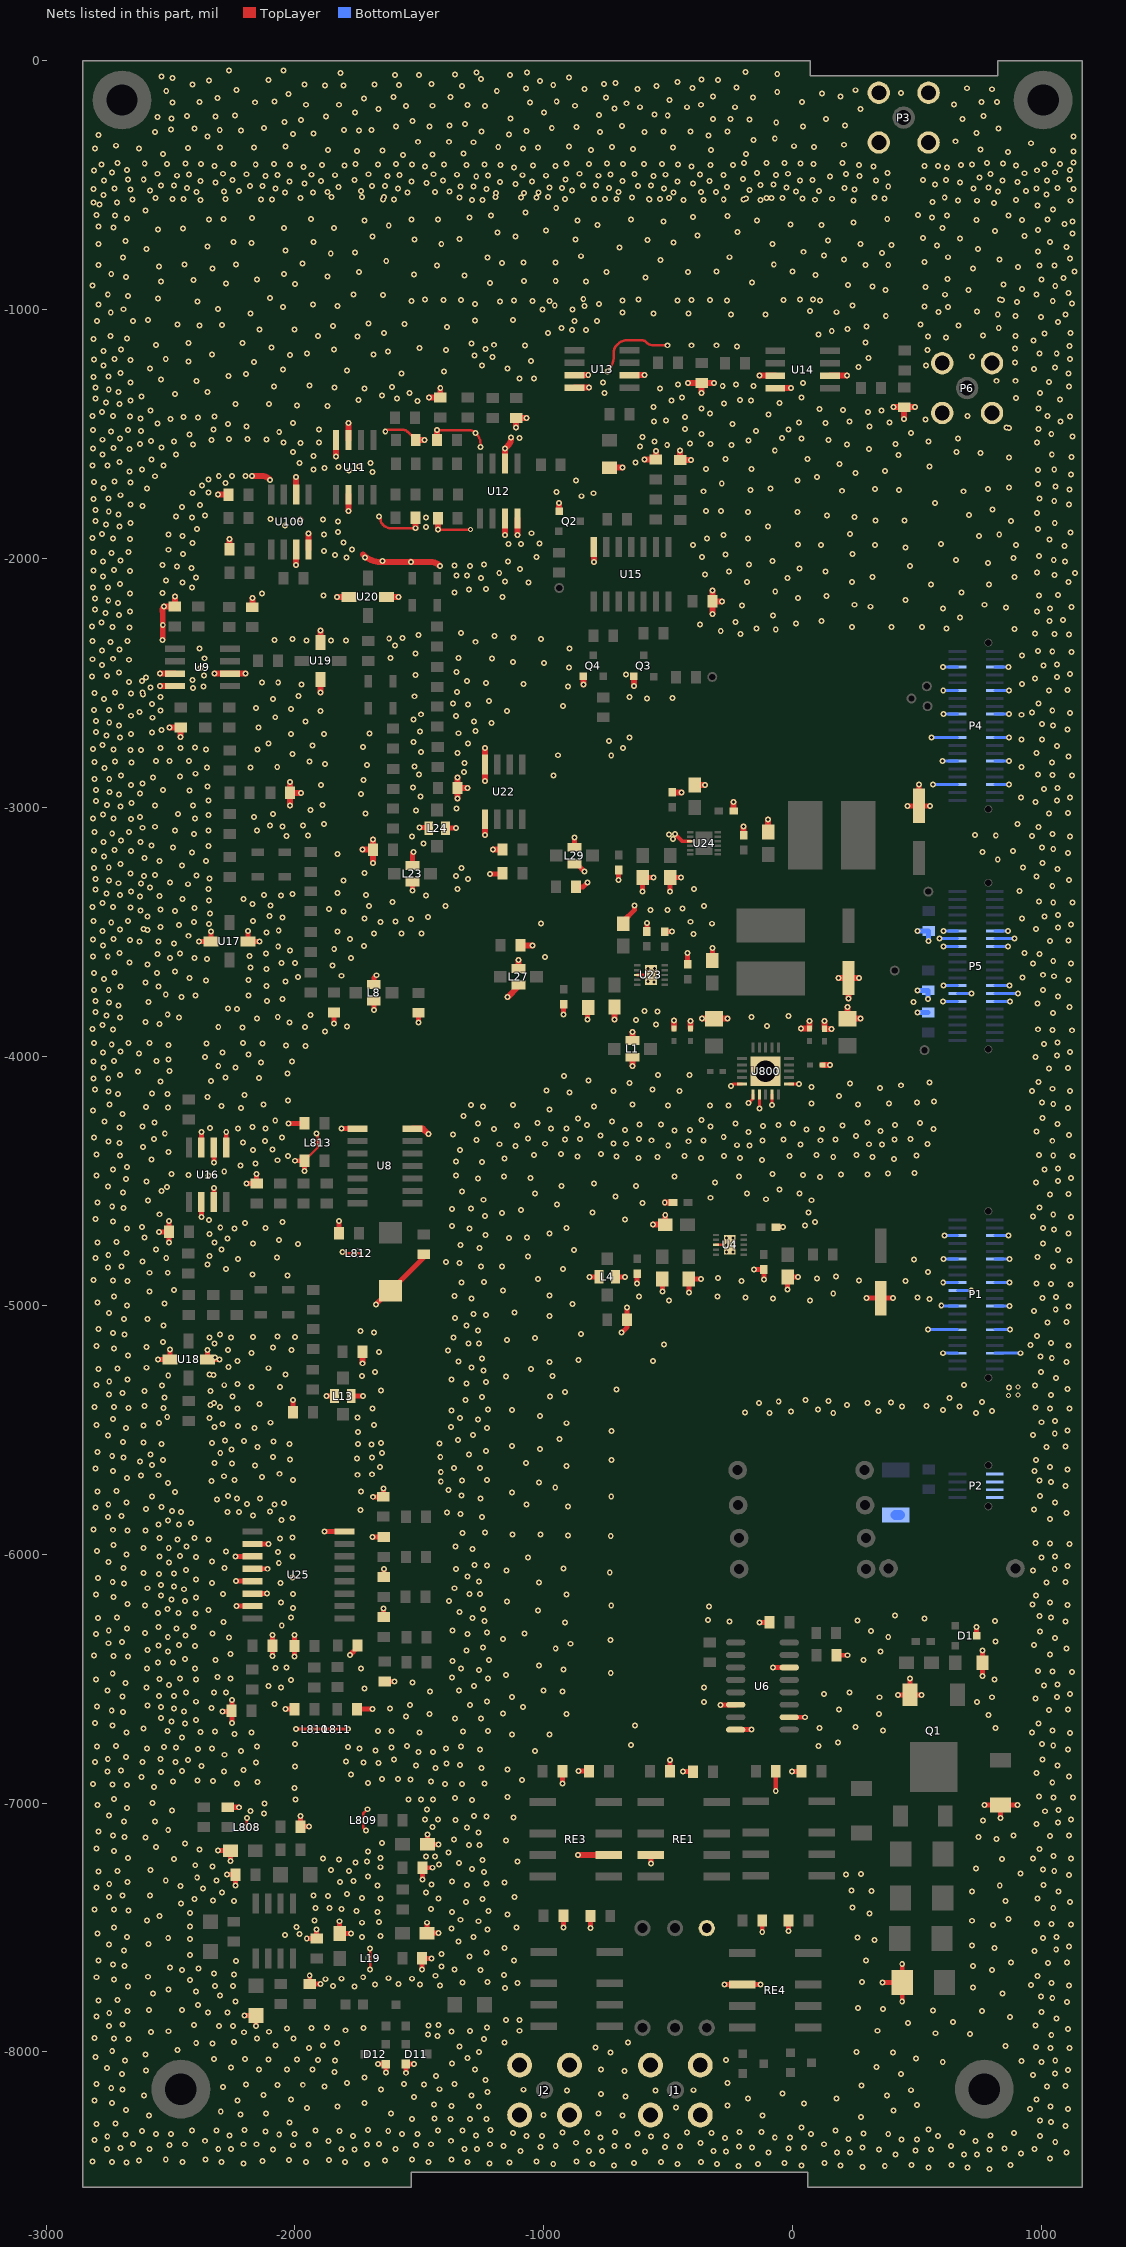
[diagram p0: the nets of this part, all layers, seen from the top]
# Altium PCB MISC109560.PcbDoc (part 4 of 7)
Units mil, origin at the board's own origin, x right, y up, seen from the top; angles counter-clockwise.
Board outline 4015.75 x 8543.31 mil, 4 copper layers (TopLayer, GND, SIG3, BottomLayer); 280 components, 173 nets, 936 pads, 3695 vias.

## Via types
v1: diameter 24, hole 12, TopLayer to BottomLayer, 3659 vias
v2: diameter 20, hole 12, TopLayer to BottomLayer, 32 vias
v3: diameter 40, hole 20, TopLayer to BottomLayer, 4 vias

## Nets (pads, with @x,y where several pads share a name; then routed paths per layer and width w, separated by ;. In a path a pad name is that pad's centre, name@x,y a point inside that pad or via, vN(x,y) a via of type N, cw(c..) or ccw(c..) an arc to the next point about the centre after c; other vN are vias at no path point) (continued)
GND: (continued)
  other v1: 790,-8471 545,-8464 702,-8464 280,-8463 370,-8459 -217,-8458 -717,-8457 35,-8456 192,-8456 478,-8455 638,-8455 875,-8455 -462,-8451 -305,-8451 -140,-8451 -1711,-8450 -962,-8450 -805,-8450 -2207,-8449 -1218,-8449 -32,-8447 128,-8447 -637,-8446 -2677,-8445 -1137,-8445 -1956,-8443 -1799,-8443 -2735,-8442 -2452,-8442 -2295,-8442 -1463,-8442 -1306,-8442 -529,-8442 -369,-8442 -2813,-8441 -1029,-8441 -869,-8441 -2131,-8438 -2627,-8437 -1638,-8437 -2023,-8434 -1863,-8434 -2519,-8433 -2359,-8433 -1530,-8433 -1370,-8433 1034,-8429 413,-8413 740,-8413 689,-8412 918,-8409 -97,-8405 230,-8405 1101,-8405 179,-8404 -594,-8400 -267,-8400 -1094,-8399 -767,-8399 -318,-8399 -818,-8398 494,-8396 555,-8393 791,-8393 -2088,-8392 -1761,-8392 346,-8392 -2755,-8391 -2584,-8391 -2257,-8391 -1812,-8391 -1595,-8391 -1268,-8391 971,-8391 -2308,-8390 -1319,-8390 -16,-8388 851,-8388 -2700,-8386 45,-8385 281,-8385 -164,-8384 -513,-8383 -1013,-8382 -452,-8380 -216,-8380 -952,-8379 -716,-8379 -661,-8379 636,-8379 -1161,-8378 -2007,-8375 -2503,-8374 -1514,-8374 -1946,-8372 -1710,-8372 -2442,-8371 -2206,-8371 -2155,-8371 -1453,-8371 -1217,-8371 126,-8371 -2651,-8370 -1662,-8370 -371,-8366 -871,-8365 1055,-8362 -1865,-8358 735,-8358 -2361,-8357 -1372,-8357 -2806,-8353 438,-8352 500,-8351 225,-8350 -272,-8345 -772,-8344 -72,-8344 -10,-8343 -2754,-8340 -569,-8339 -1069,-8338 -507,-8338 -1766,-8337 -1007,-8337 583,-8337 994,-8337 -2262,-8336 -1273,-8336 794,-8335 -2680,-8332 -2063,-8331 -2559,-8330 -2001,-8330 -1570,-8330 -2497,-8329 -1508,-8329 73,-8329 384,-8329 -624,-8327 284,-8327 -1124,-8326 -326,-8325 889,-8325 -826,-8324 -424,-8324 683,-8324 -924,-8323 -213,-8322 -713,-8321 -126,-8321 -2118,-8319 -2614,-8318 -1625,-8318 -1820,-8317 -2316,-8316 -1918,-8316 -1327,-8316 173,-8316 -2414,-8315 -1425,-8315 -1707,-8314 -2203,-8313 -1214,-8313 546,-8311 36,-8303 1097,-8297 -2797,-8289 -2721,-8287 -2022,-8284 1038,-8281 993,-8275 -1231,-8270 -1530,-8269 -1374,-8269 -1296,-8269 -1440,-8268 275,-8262 -2587,-8256 -683,-8256 -121,-8256 -1002,-8254 -2218,-8251 -1613,-8248 -2117,-8247 -780,-8247 -2298,-8240 406,-8235 -2679,-8234 1106,-8230 953,-8229 -1951,-8225 -468,-8223 -1828,-8220 1035,-8220 -1261,-8219 -1370,-8218 -261,-8216 500,-8214 -1442,-8212 45,-8208 -2735,-8206 -1720,-8205 -2806,-8196 -2230,-8196 -2016,-8192 979,-8192 -180,-8187 176,-8187 -1522,-8181 -672,-8180 -2607,-8175 -1291,-8175 379,-8175 -2126,-8173 -771,-8170 -41,-8167 -1227,-8161 -906,-8156 -551,-8155 -399,-8154 475,-8154 -1081,-8152 -2693,-8151 -1653.48,-8151 -1418.48,-8150 -2738,-8145 -2288.48,-8141 -1881.48,-8139 1021,-8139 1097,-8137 277,-8135 -2069.48,-8133 -1968.48,-8132 -2197.48,-8130 -1480.48,-8130 -2797,-8129 -1562.48,-8129 -1358,-8129 -261,-8125 -1791.48,-8124 -1234,-8112 -1719.48,-8103 -1432.48,-8096 966,-8092 -2694,-8089 435,-8088 1054,-8086 -1840.48,-8080 -675,-8076 -2598,-8074 1106,-8073 -770,-8071 -2143.48,-8070 -2031.48,-8070 -1928.48,-8070 -1277,-8070 -2755,-8064 -2256.48,-8063 336,-8061 -1368,-8046 603,-8040 1000,-8040 919,-8037 -1838.48,-8035 1055,-8035 -2682,-8034 -267,-8033 -1906.48,-8032 -2106.48,-8031 -1991.48,-8031 -2201.48,-8029 -2325.48,-8028 495,-8027 -1306,-8025 -2801,-8021 -2601,-8010 -732,-8003 404,-8002 -1260,-8001 257,-8000 -2734,-7997 -2472,-7992 -1942.48,-7985 1113,-7985 1035,-7984 -793,-7983 977,-7981 -1339,-7978 856,-7976 -2077.48,-7975 -1887.48,-7975 -2330.48,-7966 -2396.48,-7964 -1831.48,-7964 -1158,-7963 -662,-7963 -2244.48,-7961 -2669,-7949 -1241,-7948 -2005.48,-7947 -2727,-7946 -2152.48,-7946 -2805,-7945 -1427.48,-7936 1039,-7932 -1465.48,-7930 713,-7928 574,-7925 -2205,-7921 -2578,-7920 -2104,-7919 -1370,-7918 -2508,-7917 -1297,-7916 -1098,-7915 340,-7915 -1797.48,-7913 1106,-7908 -2032.48,-7905 -1932.48,-7903 -1724.48,-7903 -1871.48,-7902 -1228,-7901 -2747,-7895 -2304.48,-7895 -2248.48,-7895 976,-7894 -1463.48,-7893 -2405.48,-7892 -1423.48,-7891 -2692,-7890 464,-7884 645,-7880 -1097,-7872 -1152,-7871 1060,-7865 873,-7859 -2798,-7857 -2746,-7844 -2349.48,-7842 -2270.48,-7842 999,-7840 -2672,-7836 761,-7836 564,-7833 -2454,-7832 -2586,-7831 362,-7827 263,-7824 -2389.48,-7812 1102,-7800 -2238.48,-7798 -2789,-7793 -2713,-7791 1043,-7784 998,-7778 -2300.48,-7773 -2571,-7766 844,-7766 -2397.48,-7757 -2507,-7749 -1155,-7743 724,-7741 -2671,-7738 -1761.48,-7737 -2320.48,-7735 -2248.48,-7735 -1847.48,-7735 -1417.48,-7734 1111,-7733 958,-7732 -1677.48,-7730 -1496.48,-7730 -1583.48,-7728 -1106,-7723 1040,-7723 -1327,-7721 279,-7720 -1227,-7719 -2421,-7712 -2727,-7710 -1876.48,-7708 -1812.48,-7706 -1529.48,-7706 -1624.48,-7704 -2798,-7700 -1725.48,-7700 -2591,-7698 984,-7695 -1434.48,-7694 -1160,-7691 -2245.48,-7689 -2325.48,-7685 -2453,-7671 -1255,-7670 800,-7670 -1358,-7669 -2387,-7664 -2502,-7660 -1410.48,-7657 -2685,-7655 724,-7655 -2730,-7649 1026,-7642 878,-7641 1102,-7640 -2237.48,-7635 -2789,-7633 -1119,-7633 294,-7633 -1299,-7616 -2422.48,-7611 -1411.48,-7607 -1230,-7601 971,-7595 -2686,-7593 1059,-7589 -1158,-7583 810,-7582 1111,-7576 720,-7572 -2747,-7568 -2589,-7566 -1343,-7557 329,-7550 -2422.48,-7547 1005,-7543 -2509,-7542 261,-7541 -2674,-7538 -1730.48,-7538 -1282,-7538 1060,-7538 -1655.48,-7534 -2040.48,-7530 -1981.48,-7527 -2793,-7525 -1226,-7509 -1370,-7505 -2726,-7501 -1110,-7500 -1994.48,-7499 -2422.48,-7497 804,-7490 1118,-7488 1040,-7487 982,-7484 -1730.48,-7481 -1661.48,-7478 -1262,-7475 720,-7473 -2594,-7472 -1920.48,-7472 -1334,-7469 867,-7466 -2544,-7453 -1146,-7448 309,-7443 -2422.48,-7442 -1369,-7438 -1667.48,-7437 -1222,-7434 -1753.48,-7433 -2669,-7431 -2727,-7428 -2805,-7427 -1453.48,-7426 -1812.48,-7425 -1861.48,-7422 1047,-7422 -1917.48,-7421 240,-7420 -2457,-7404 1114,-7398 -1313,-7397 855,-7394 -2244.48,-7393 -2329.48,-7391 -2403.48,-7386 -1247,-7385 -1656.48,-7384 -1423.48,-7384 984,-7384 -1730.48,-7382 -2747,-7377 -1117,-7377 -1866.48,-7374 -2692,-7372 -2583,-7371 -1925.48,-7371 -1790.48,-7366 -2293.48,-7360 -1473.48,-7359 720,-7356 1068,-7355 317,-7353 236,-7352 -2368.48,-7343 -2798,-7339 -2460,-7334 -1667.48,-7332 832,-7331 -1308,-7330 1007,-7330 -1451.48,-7328 -2746,-7326 -1230,-7324 -1158,-7319 -2672,-7318 -1819.48,-7317 -1368,-7315 -1765.48,-7313 -2519,-7312 -2314.48,-7311 -2392.48,-7300 -1706.48,-7295 1110,-7290 214,-7287 275,-7286 915,-7284 -1240,-7278 -2789,-7275 1051,-7274 -2713,-7273 -1783.48,-7273 -2581,-7269 -1855.48,-7269 1006,-7268 -1289,-7266 737,-7263 -1656.48,-7258 -2331.48,-7255 -2400.48,-7250 -1421,-7247.31 -1341,-7241 -1756.48,-7239 -1709.48,-7235 -1106,-7234 -1247,-7229 -1823.48,-7226 842,-7225 -2485,-7224 1119,-7223 -1886.48,-7222 966,-7222 -2671,-7220 -1656.48,-7220 -1473.48,-7215 -1437.48,-7214 1048,-7213 -1382,-7198 -1707,-7195 -2727,-7192 -2383,-7187 992,-7185 -2798,-7182 -2559,-7176 -1300,-7169 -1259,-7169 -2442,-7163 -1651,-7161 -1152,-7151 -1361,-7146 819,-7144 -2601,-7139 -2685,-7137 747,-7136 1034,-7132 -2730,-7131 888,-7130 1110,-7130 -1263,-7118 -2789,-7115 -2509,-7109 -1309,-7098 -1447.48,-7096 979,-7085 1067,-7079 -2686,-7075 -2563,-7075 764,-7070 -1354,-7068 -1477.48,-7066 -1424.48,-7066 1119,-7066 -1121,-7059 -1231,-7055 -1280,-7052 -2747,-7050 -2125,-7042 1013,-7033 -2178,-7032 -2494,-7030 1068,-7028 -1468.48,-7026 -2674,-7020 -2793,-7007 -2122,-7001 -2573,-6999 -1288,-6988 -1998,-6986 -1544.48,-6986 -1492.48,-6986 -1445.48,-6985 -2726,-6983 -1357,-6979 1126,-6978 1048,-6977 -1146,-6976 990,-6974 -2001,-6940 -2567,-6936 -2675,-6928 -2733,-6925 -2811,-6924 -1329,-6924 -1397,-6923 -2233,-6922 -1239,-6922 -1707,-6919 1043,-6917 -2151,-6916 -2490,-6914 -1454,-6914 -2329,-6912 -2392,-6910 -1088,-6908 -1536,-6905 -1650,-6904 -1586,-6903 -2616,-6896 1110,-6893 -1774,-6886 980,-6879 -2539,-6875 -2753,-6874 -2284,-6873 -2453,-6871 -2698,-6869 -2206,-6867 -1146,-6866 -1251,-6860 -1436,-6859 -2000,-6854 -2376,-6851 -1514,-6850 1064,-6850 -1337,-6847 -1390,-6842 -1665,-6839 -1724,-6838 -2157,-6837 -2804,-6836 -2612,-6835 -2480,-6835 -1795,-6834 -2429,-6828 -1601,-6826 1003,-6825 -2541,-6824 -2752,-6823 -2678,-6815 -2282,-6806 -1503,-6795 -1446,-6795 -1036,-6791 -2217,-6790 -1677,-6788 -1257,-6785 1106,-6785 -2390,-6782 -2594,-6781 -2333,-6781 -1741,-6781 -1392,-6781 -2477,-6777 -1611,-6776 -2526,-6775 -1786,-6774 -2153,-6773 -1333,-6773 -2795,-6772 -1550,-6771 103,-6771 -2719,-6770 1047,-6769 -649,-6767 -1999,-6763 1002,-6763 183,-6757 -2453,-6737 -1127,-6725 -977,-6725 -2242,-6722 1115,-6718 -2677,-6717 -2174,-6717 962,-6717 -1499,-6716 -2380,-6715 -2320.93,-6712.01 -1325,-6712 -2511.93,-6711.01 -1666,-6710 -1611,-6710 -1225,-6710 363,-6708 1044,-6708 -2609,-6700 107,-6698 815,-6698 253,-6694 -2733,-6689 -634,-6688 -2440.93,-6680.01 988,-6680 -2804,-6679 -2495.93,-6673.01 -2396.93,-6666.01 -1253,-6661 -1356,-6660 -2538.93,-6658.01 -1554,-6653 786,-6647 -1460,-6643 -909,-6642 347,-6642 -1163,-6641 -2691,-6634 -2445.93,-6632.01 -2736,-6628 1030,-6627 186,-6625 1106,-6625 -2484.93,-6621.01 -1618,-6620 -2334.93,-6618.01 -1083,-6615 -2538.93,-6614.01 -2795,-6612 -2592,-6608 -1297,-6607 -1538,-6606 -2082,-6603 -356,-6595 740,-6595 -2397.93,-6593.01 -1228,-6592 975,-6580 348,-6575 800,-6575 -1128,-6574 1063,-6574 -2692,-6572 -2545.93,-6570.01 -2485.93,-6569.01 125,-6562 1115,-6561 228,-6556 -2437.93,-6555.01 -2324.93,-6555.01 -2277,-6555 -925,-6552 -1458,-6551 -1341,-6548 -2753,-6547 -1002,-6547 -1721,-6539 -2597,-6535 -2055,-6535 -356,-6535 -2107,-6530 -1280,-6529 1009,-6528 -2505.93,-6525.01 1064,-6523 -2680,-6517 -1528,-6516 -2016,-6505 -2799,-6504 -2396.93,-6503.01 810,-6503 -2544.93,-6501.01 -2258.93,-6500.01 -1224,-6500 -2461.93,-6499.01 -1368,-6496 -2310.93,-6494.01 -1151,-6486 -2732,-6480 -731,-6478 1122,-6473 1044,-6472 986,-6469 -1260,-6466 -921,-6463 -1332,-6460 -2594,-6459 -2401.93,-6459.01 -1735,-6459 -2078.93,-6457.01 -2033.93,-6455.01 -1020,-6448 -2549.93,-6436.01 -2489.93,-6435.01 -1367,-6429 -2319.93,-6425.01 -1220,-6425 284,-6425 -2441.93,-6421.01 -2671,-6412 -2729,-6409 -2807,-6408 1033,-6403 -2257.93,-6401.01 353,-6392 -2509.93,-6391.01 -1311,-6388 -2592,-6386 -952,-6380 1100,-6379 -1245,-6376 -2400.93,-6369.01 -2548.93,-6367.01 -2465.93,-6365.01 970,-6365 -893,-6360 -2749,-6358 -2694,-6353 814,-6351 -732,-6345 -1163,-6341 1054,-6336 -2264.93,-6334.01 -2510.93,-6332.01 384,-6332 -2439.93,-6327.01 -1306,-6321 -2800,-6320 -2331.93,-6319.01 -1077,-6318 -2602,-6317 -1228,-6315 993,-6311 315,-6309 -2748,-6307 -1366,-6306 -2674,-6299 -2475.93,-6298.01 -2547.93,-6293.01 -2407.93,-6293.01 -2052.93,-6286.01 -914,-6275 -2286.93,-6273.01 1096,-6271 -254,-6270 -1238,-6269 812,-6268 261,-6266 -341,-6265 529,-6258 -1287,-6257 -2791,-6256 1037,-6255 -2715,-6254 -2014.93,-6254.01 992,-6249 412,-6246 -2398.93,-6239.01 -2467.93,-6237.01 -2550.93,-6236.01 -1339,-6232 -1023,-6226 -2346.93,-6224.01 -2511.93,-6220.01 -1245,-6220 -2007.93,-6216.01 -336,-6211 -2602,-6207 -729,-6207 1105,-6204 964,-6203 -2673,-6201 -2055.93,-6195.01 1034,-6194 -1147,-6191 -2440.93,-6189.01 -1380,-6189 -2495.93,-6182.01 -2396.93,-6175.01 -2729,-6173 -2538.93,-6167.01 978,-6166 -2800,-6163 -909,-6162 -2288.93,-6161.01 -2007.93,-6161.01 -1298,-6160 -1257,-6160 -2445.93,-6141.01 -2592,-6137 -1359,-6137 -2484.93,-6130.01 -2538.93,-6123.01 -2687,-6118 -2332.93,-6116.01 -2057.93,-6116.01 -1019,-6113 1020,-6113 -2732,-6112 1096,-6111 -1261,-6109 -2397.93,-6102.01 -2791,-6096 -2008.93,-6094.01 -1307,-6089 -2545.93,-6079.01 -2485.93,-6078.01 -2609,-6076 -735,-6073 965,-6066 -1150,-6065 -2437.93,-6064.01 1053,-6060 -1352,-6059 -920,-6057 -2688,-6056 -2282.93,-6056.01 1105,-6047 -1229,-6046 -1278,-6043 -2064.93,-6035.01 -2505.93,-6034.01 -2749,-6031 -2332.93,-6030.01 -1064,-6014 999,-6014 -2396.93,-6012.01 -2544.93,-6010.01 -2008.93,-6009.01 1054,-6009 -2461.93,-6008.01 -2676,-6001 -2067.93,-5992.01 -2276.93,-5989.01 -2795,-5988 -1286,-5979 -2608,-5975 -2506.93,-5975.01 -2435.93,-5970.01 -1355,-5970 -2728,-5964 1112,-5959 1034,-5958 976,-5955 -2471.93,-5941.01 -2347.93,-5941.01 -2059.93,-5937.01 -2543.93,-5936.01 -2403.93,-5936.01 -2008.93,-5934.01 -731,-5927 -903,-5926 -1126,-5921 -1013,-5921 -1327,-5915 -1237,-5913 -2673,-5905 -2601,-5905 -2731,-5902 -2809,-5901 -2465.93,-5881.01 -2548.93,-5880.01 -2418,-5875 -2509.93,-5864.01 -2053.93,-5862.01 1033,-5859 -2009.93,-5855.01 -2751,-5851 -1249,-5851 -2696,-5846 -2168.93,-5844.01 -1335,-5838 1100,-5835 -1388,-5833 -2457,-5831 -2223.93,-5831.01 -2270.93,-5830.01 -2100,-5829 -2493.93,-5826.01 -1737,-5823 970,-5821 -2599,-5819 -2802,-5813 -2536.93,-5811.01 -903,-5808 -2750,-5800 -2082.93,-5800.01 -1069,-5800 -2191.93,-5798.01 -2043.93,-5795.01 -2676,-5792 1054,-5792 -2312.93,-5780.01 -2231.93,-5776.01 -2139.93,-5776.01 -1255,-5776 -2574,-5768 -729,-5768 993,-5767 -2268.93,-5766.01 -1331,-5764 -1128,-5752 -2481,-5750 -2793,-5749 -1734,-5748 -2717,-5747 -1382,-5742 -954,-5733 1096,-5727 -2510,-5714 -1019,-5712 1037,-5711 -1414,-5709 -2335,-5707 -1329,-5705 992,-5705 -2008,-5703 -1229,-5703 -2242,-5702 -2675,-5694 -2132,-5690 -2285,-5687 -2619,-5684 -2549,-5683 -1748,-5681 -1691,-5679 -2061,-5677 -1414,-5669 -2731,-5666 971,-5666 1105,-5660 -2802,-5656 -1257,-5654 -1360,-5653 -1659,-5650 1034,-5650 -909,-5645 -2161,-5643 -2574,-5641 -2252,-5636 -1072,-5634 -2324,-5633 -2622,-5627 978,-5622 -2530,-5621 -728,-5621 -2019,-5619 -1751,-5616 -1690,-5612 -2689,-5611 -1416,-5610 -2088,-5609 -2734,-5605 -2580,-5600 -1301,-5600 -2300,-5594 -1651,-5594 -2793,-5589 -1232,-5585 -2255,-5579 -1016,-5578 -2151,-5570 1020,-5569 1096,-5567 -1128,-5565 -1693,-5560 -2021,-5558 -1746,-5558 -2537,-5557 -1419,-5555 -1654,-5554 -2334,-5553 -2609,-5551 -2690,-5549 -2086,-5547 -2205,-5546 -2281,-5544 -1345,-5541 -936,-5538 -2751,-5524 -1284,-5522 965,-5522 1053,-5516 -1747,-5509 -728,-5506 1105,-5503 -2678,-5494 -2163,-5493 -1228,-5493 -2323.96,-5488.31 -1372,-5489 -2227.96,-5485.31 -2608,-5483 -2797,-5481 -1682,-5481 -2290.96,-5477.31 -909,-5474 -2546.96,-5472.31 -2098,-5472 999,-5470 1054,-5465 -1264,-5459 -2730,-5457 -2343.96,-5452.31 -1336,-5453 -1748,-5451 -2512.96,-5448.31 -1016,-5444 -93,-5433 163,-5433 736,-5433 -191,-5431 -7,-5427 800,-5425 344,-5424 -1371,-5422 604,-5421 -1128,-5420 102,-5419 -1224,-5418 -2230.96,-5415.31 1112,-5415 -1688,-5414 1034,-5414 -2527.96,-5412.31 -2669,-5412 976,-5411 -2727,-5409 -2300.96,-5408.31 -2805,-5408 440,-5407 671,-5407 -2604,-5405 537,-5404 -2339.96,-5401.31 218,-5401 -2142,-5397 -2324.96,-5392.31 -135,-5393 301,-5392 395,-5391 760,-5388 -56,-5387 143,-5385 -1315,-5381 51,-5381 -2523.96,-5371.31 630,-5372 -1249,-5369 -2250.96,-5367.31 -976,-5367 1037,-5360 -2747,-5358 -2692,-5353 -914,-5348 -2338.96,-5345.31 -2604,-5344 -1654,-5343 -708,-5338 1104,-5336 869,-5330 -2174,-5328 -2059,-5328 -2534.96,-5322.31 -2283.96,-5321.31 974,-5322 689,-5321 -2798,-5320 -2229.96,-5316.31 -1310,-5314 -1232,-5308 -2746,-5307 -2672,-5299 -1370,-5299 1058,-5293 -1152,-5286 -1731,-5285 -965,-5284 -2508.96,-5281.31 -2326.96,-5279.31 -2342.96,-5278.31 -2037,-5279 -1678,-5268 997,-5268 -1242,-5262 -1051,-5257 -2789,-5256 -2713,-5254 -2107,-5253 -2596,-5251 -1291,-5250 -2265.96,-5247.31 1100,-5228 -978,-5227 -1343,-5225 -2230.96,-5223.31 -562,-5223 -861,-5219 -1249,-5213 1041,-5212 -2321.96,-5209.31 996,-5206 -2671,-5201 -2174,-5191 -1662,-5188 -1384,-5182 -2268.96,-5180.31 -2013,-5179 -2727,-5173 -2088,-5170 -2596,-5168 -2798,-5163 1109,-5161 956,-5160 -517,-5158 -2322.96,-5153.31 -1302,-5153 -1261,-5153 1038,-5151 -2529.96,-5148.31 -1147,-5139 -1035,-5131 -2342.96,-5129.31 -2255.96,-5129.31 -1363,-5130 -2168,-5127 -2000,-5127 -2070,-5125 982,-5123 -2685,-5118 -2301.96,-5117.31 -850,-5115 -2730,-5112 -1682,-5110 -1737,-5104 -1265,-5102 -2789,-5096 -2527.96,-5081.31 -1311,-5082 1024,-5070 1100,-5068 -2686,-5056 -2592,-5055 -1356,-5052 -978,-5043 -1233,-5039 -1282,-5036 -2747,-5031 -1118,-5029 969,-5023 1057,-5017 1109,-5004 -2674,-5001 -885,-4994 -2524,-4992 -2793,-4988 -497,-4981 70,-4980 549,-4974 -80,-4973 -1290,-4972 1003,-4971 -189,-4969 501,-4969 1058,-4966 -2726,-4964 -618,-4964 -302,-4964 -1359,-4963 -977,-4961 163,-4953 -2585,-4945 -1163,-4941 -2485,-4938 1116,-4916 1038,-4915 980,-4912 -1331,-4908 -1241,-4906 -2673,-4903 -206,-4902 454,-4902 266,-4901 -2731,-4900 -2809,-4899 -1024,-4895 98,-4893 -301,-4891 175,-4885 -2030,-4880 -2171,-4876 -2583.96,-4869.31 -2510.96,-4869.31 543,-4867 -2277,-4855 -922,-4855 -2751,-4849 -1168,-4845 -2696,-4844 -1253,-4844 1046,-4844 -2351.96,-4836.31 -1339,-4831 -1392,-4826 -2611.96,-4823.31 1113,-4820 486.92,-4816 -2228,-4815 -2802,-4811 -2516.96,-4809.31 -2072,-4808 983,-4806 -1064,-4804 -2342.96,-4801.31 -2750,-4798 -2676,-4790 -1808,-4786 -879,-4778 1067,-4777 -2558.96,-4775.31 -2294.96,-4775.31 -1259,-4769 -1335,-4757 -1988,-4754 -2169,-4752 1006,-4752 -2323.96,-4748.31 -2793,-4747 -2717,-4745 -2064,-4737 -2270.96,-4731.31 -1139,-4729 -2604.96,-4727.31 -1067,-4727 -1235,-4717 -2343.96,-4713.31 1109,-4712 -978,-4711 1050,-4696 -2241.96,-4692.31 -2675,-4692 -1298,-4691 -2119,-4690 1005,-4690 -2299.96,-4688.31 -909,-4689 -2613.96,-4686.31 -1368,-4681 50,-4679 -2200.96,-4669.31 90,-4666 -2049,-4665 -2731,-4664 -2344.96,-4657.31 -673,-4655 -2802,-4654 1118,-4645 965,-4644 -1236,-4641 -2544.96,-4634.31 1047,-4635 -1168,-4630 -804,-4628 63,-4628 -1091,-4617 -1368,-4613 -1292,-4611 -2689,-4609 991,-4607 -2734,-4603 -946,-4596 -604,-4590 -2793,-4587 -2589.96,-4579.31 76,-4578 -1243,-4576 -108,-4574 -331,-4568 -711,-4563 1033,-4554 1109,-4552 -183,-4551 27,-4551 -1035,-4550 -2690,-4547 -1328,-4542 -2536.96,-4540.31 -52,-4534 -2513.96,-4525.31 -2751,-4522 -928,-4521 -630,-4521 -799,-4510 -313,-4507 978,-4507 -2595.96,-4503.31 1066,-4501 -2678,-4492 -1264,-4490 -1053,-4489 1118,-4488 110,-4485 -1160,-4483 -475,-4483 -215,-4482 -2347.96,-4479.31 -2797,-4479 -1353,-4478 -2427.96,-4476.31 42,-4476 -2495.96,-4473.31 194,-4474 300,-4474 -82,-4472 383,-4471 489,-4468 -2283.96,-4462.31 -2730,-4455 1012,-4455 1067,-4450 -2675,-4444 -2218.96,-4439.31 -2157.96,-4430.31 -1249,-4424 -1353,-4423 -2069.96,-4417.31 -123,-4416 -2576.96,-4414.31 408,-4412 -1158,-4411 -619,-4409 -368,-4409 -211,-4409 163,-4405 320,-4405 -543,-4404 -864,-4402 -707,-4402 -2026.96,-4399.31 -435,-4400 -275,-4400 -12,-4400 1125,-4400 1047,-4399 -2702,-4398 498,-4398 -1039,-4397 96,-4396 256,-4396 989,-4396 -2797,-4394 -931,-4393 -771,-4393 -2507.96,-4383.31 -2167.96,-4375.31 -1336,-4376 -2089.96,-4374.31 -2609.96,-4363.31 -1113,-4360 -500,-4358 -173,-4358 -224,-4357 31,-4354 358,-4354 -1178,-4353 307,-4353 541,-4352 -996,-4351 -669,-4351 -720,-4350 -2704,-4348 -2208.96,-4346.31 -2749,-4342 -419,-4341 -2119.96,-4339.31 1043,-4339 -358,-4338 -122,-4338 -567,-4337 112,-4337 -1271,-4335 -915,-4334 173,-4334 409,-4334 -2566.96,-4332.31 -36,-4333 -854,-4331 -618,-4331 474,-4331 -1063,-4330 -2050.96,-4326.31 -2808,-4326 -277,-4324 254,-4320 -773,-4317 1110,-4315 -1364,-4314 -2522.96,-4310.31 -178,-4303 980,-4301 353,-4299 -475,-4297 -674,-4296 -413,-4296 56,-4293 -1200,-4292 118,-4292 -2228.96,-4290.31 -2117.96,-4290.31 566,-4291 -971,-4290 -909,-4289 -2340.96,-4287.31 -2705,-4286 -2170.96,-4284.31 -2611.96,-4281.31 -330,-4282 -119,-4280 -1108,-4278 201,-4278 412,-4276 -826,-4275 -57,-4275 -529,-4274 -615,-4273 1064,-4272 -1264,-4270 2,-4270 -230,-4269 512,-4268 -2563.96,-4266.31 -1025,-4267 301,-4265 -726,-4262 -2766,-4261 -2079,-4258 -367,-4256 -863,-4249 1003,-4247 -1323,-4239 -2693,-4231 -2812,-4218 -978,-4213 -2217,-4207 1106,-4207 -2510,-4206 -2599,-4204 -1245,-4202 -799,-4201 -2295,-4200 -501,-4198 -332,-4198 -257,-4197 -1293,-4195 -1124,-4195 -2745,-4194 -2126,-4194 -644,-4194 262,-4193 1047,-4191 75,-4189 387,-4189 499,-4186 1002,-4185 568,-4182 -2027,-4178 -2352,-4164 187,-4159 -2202,-4155 -2710,-4151.31 -2512,-4152 -2574,-4149 -896,-4145 -2749,-4140.31 1115,-4140 -719,-4139 -455,-4139 962,-4139 -990,-4138 -2803,-4133.31 -563,-4133 1044,-4130 351,-4127 76,-4123 436,-4116 230,-4108 -656,-4107 549,-4104 988,-4102 -2540,-4101 -2338,-4099 -820,-4096 -2810,-4089.31 -2750,-4088.31 -2144,-4086 -2279,-4084 -918,-4079 -2702,-4074.31 -541,-4075 -415,-4075 -2030,-4069 -2630,-4061 -2504,-4059 1030,-4049 1106,-4047 -2770,-4044.31 -2238,-4044 -2308,-4038 -2137,-4024 -2809,-4020.31 -2011,-4021 -2726,-4018.31 -2557,-4019 -2508,-4013 -2361,-4002 975,-4002 1063,-3996 -2186,-3992 -2626,-3989 -2771,-3985.31 -2291,-3985 1115,-3983 -2700,-3980.31 -1957,-3958 -2035,-3956 -2508,-3954 -2736,-3951.31 1009,-3950 -2355,-3949 -2131,-3949 -2808,-3946.31 -2668,-3946.31 -2584,-3947 -2209,-3947 1064,-3945 -1880,-3899.31 1122,-3895 1044,-3894 -2730,-3891.31 -2813,-3890.31 986,-3891 -2210,-3883 -2308,-3882 -1959,-3881.31 -1791,-3879 -103,-3877 -2774,-3874.31 -550,-3872 -2544,-3869.31 -2022,-3864 -2601,-3862.31 -629,-3854 -2152,-3847 -2703,-3843.31 -2466,-3844 -166,-3842 -2069,-3841 -2758,-3836.31 -16,-3837 -1937,-3834.31 -2511,-3832.31 1046,-3826 -2801,-3821.31 -543,-3819 -595,-3818 -2232,-3809 -2268,-3808 1113,-3802 -2708,-3795.31 983,-3788 -2747,-3784.31 -2589,-3781.31 486,-3781.31 -2801,-3777.31 -2112,-3777.31 -2049,-3769.31 -2456,-3761.31 1067,-3759 -2399,-3756 -2186,-3755.31 -2519,-3751.31 -2808,-3733.31 1006,-3734 -2748,-3732.31 -2548,-3719.31 -2700,-3718.31 -2114,-3716.31 -2601,-3702.31 -2037,-3698.31 -2358,-3696 1109,-3694 -2186,-3692.31 -2768,-3688.31 -2424,-3684.31 923,-3682.31 -1988,-3680.9 1050,-3678 -1813,-3676 1005,-3672 -2807,-3664.31 -2554,-3664.31 -2724,-3662.31 -2481,-3658.31 -2114,-3648.31 -2178,-3642.31 -1849,-3635.31 -2592,-3631.31 1118,-3627 965,-3626 -2054,-3624.31 -2000,-3623.9 -2664,-3622.31 1047,-3617 -2353,-3609.31 -2502,-3604.31 -2403,-3604.31 -1774,-3604.31 -996,-3601 -2812,-3599.31 -2752,-3598.31 -2182,-3596.31 -2552,-3589.31 991,-3589 -2461,-3587.31 -2117,-3587.31 931,-3585.31 -2704,-3584.31 -2020,-3574.31 -1842,-3569.31 -2067,-3558.31 -1723,-3557.31 -2772,-3554.31 -2485,-3547.31 -2549,-3539.31 -2625,-3538.31 1033,-3536 1109,-3534 -2663,-3532.31 -2811,-3530.31 -2728,-3528.31 -1778,-3528.31 -2428,-3515.31 -399,-3509 -1682,-3507 -1571,-3507 -1492,-3507 -2115,-3502.31 -1828,-3498 -2773,-3495.31 -2065,-3493.31 -2592,-3491.31 -2702,-3490.31 -2609,-3488.31 978,-3489 1066,-3483 -2540,-3479.31 -2465,-3471.31 1118,-3470 -2345,-3467.31 -324,-3467 -1012,-3466 -2738,-3461.31 -2405,-3460.31 -1656,-3460.31 -410,-3459 -1596,-3457.31 -2810,-3456.31 -2670,-3456.31 -2169,-3455.31 -1534,-3447.31 -1721,-3445.31 922,-3445.31 -2050,-3441.31 -1465,-3440.31 -2592,-3438.31 1012,-3437 -2102,-3435.31 1067,-3432 -2341,-3425.31 -1805,-3418 -2481,-3415.31 -2621,-3413.31 -572,-3412 -503,-3412 -2541,-3409.31 -1864,-3408 -442,-3406 -2403,-3404.31 -2661,-3402.31 -2730,-3400.31 -2813,-3399.31 -1703,-3395.31 -1395,-3395.31 -357,-3395 -2098,-3393.31 -2170,-3387.31 -2774,-3383.31 1125,-3382 1047,-3381 -1608,-3379 989,-3378 -2345,-3374.31 -2451,-3367.31 -2206,-3367.31 -2623,-3357.31 -2544,-3355.31 -2055,-3354.31 -1474,-3354 -2703,-3352.31 -1715,-3352.31 -2125,-3351.31 -2010,-3347.31 -2758,-3345.31 -1828,-3344 -2659,-3338.31 912,-3335.31 -2801,-3330.31 -2348,-3327.31 -1346,-3326.61 -397,-3327 -2582,-3321 1043,-3315 -2429,-3308.31 -2618,-3305.31 -2708,-3304.31 -2502,-3301.31 -2747,-3293.31 -1805,-3293 1110,-3291 -2801,-3286.31 -1305,-3286.31 -2344,-3284.31 980,-3277 -2606,-3275.31 -1352,-3276 -2395,-3273.31 -2562,-3270.31 -2660,-3265.31 -1720,-3262.31 1064,-3248 -1330,-3243.31 -2808,-3242.31 -2748,-3241.31 926,-3240.31 -2454,-3232.31 -2700,-3227.31 1003,-3223 -2545,-3215.31 -2358,-3215.31 824,-3209.31 -2605,-3203 -2768,-3197.31 -1829,-3186 1106,-3183 -2414,-3181.31 762,-3179.31 -1524,-3178.31 -2659,-3175.31 885,-3174.31 -2807,-3173.31 -2724,-3171.31 1047,-3167 -2489,-3161.31 1002,-3161 -2348,-3155.31 -2577,-3152.31 -1484,-3144.31 -2620,-3139.31 -2769,-3138.31 -2698,-3133.31 -481,-3126 -1529,-3117 1115,-3116 -2033,-3115 962,-3115 816,-3113.31 -1947,-3112.31 733,-3111.31 -2405,-3107.31 -497,-3108 1044,-3106 -2734,-3104.31 -2806,-3099.31 -2666,-3099.31 -2153,-3093.31 -2481,-3092.31 -2347,-3092.31 -2612,-3081.31 -1353,-3082 -2563,-3077.31 988,-3078 -2050,-3076.31 -2100,-3072.31 -1967,-3072.31 -1884,-3065.31 904,-3065.31 -2659,-3046.31 -2728,-3044.31